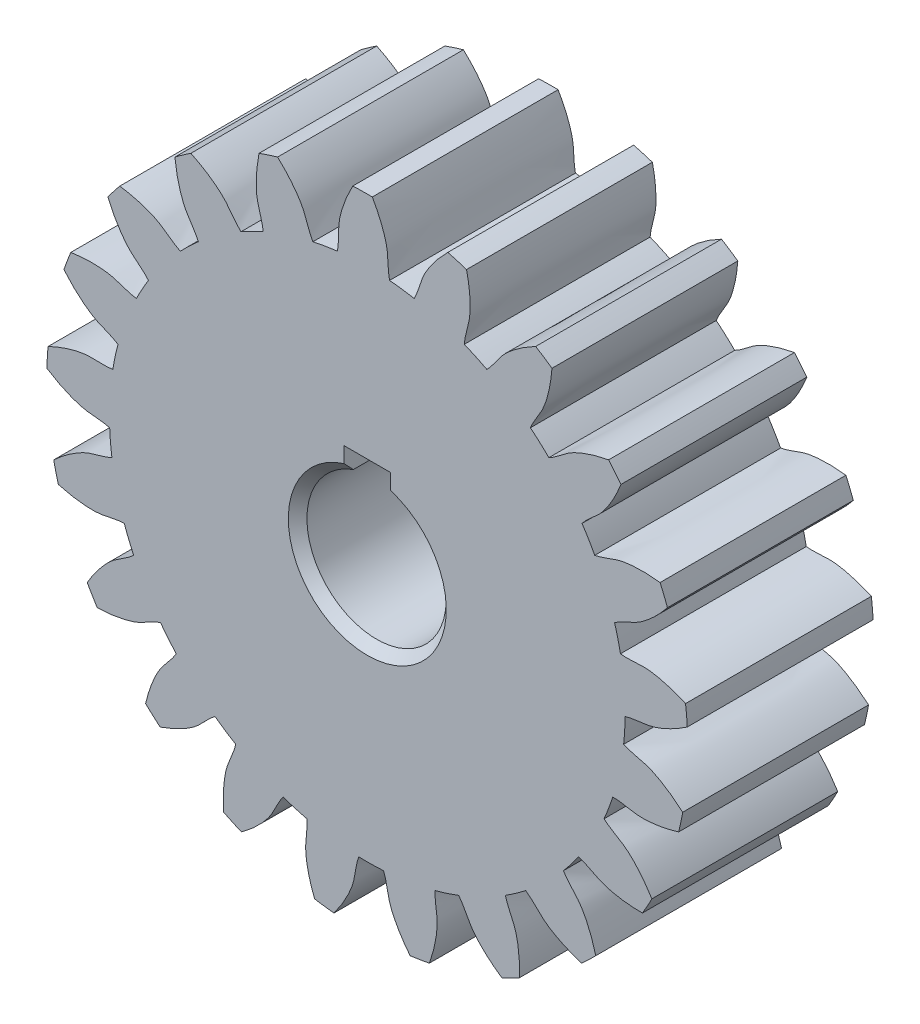
from build123d import *

# Parameters (mm, degrees)
SKETCH1_R           = 27.75
SKETCH1_R_2         = 7.5
BOSS_EXTRUDE1_DEPTH = 20
BOSS_EXTRUDE2_DEPTH = 20
CIRPATTERN1_COUNT   = 21
CHAMFER1_SIZE       = 1
CUT_EXTRUDE1_REACH  = 54.721
SKETCH3_W           = 5
SKETCH3_H           = 4.6


with BuildPart() as part:
    # Sketch1 → Boss-Extrude1 (new body)
    with BuildSketch(Plane.XY):
        Circle(SKETCH1_R)
        Circle(SKETCH1_R_2, mode=Mode.SUBTRACT)
    extrude(amount=BOSS_EXTRUDE1_DEPTH)

    # Sketch2 → Boss-Extrude2 (add)
    with BuildSketch(Plane.XY):
        with BuildLine():
            ThreePointArc((34.251201859, 4.135839847), (34.361284978, 3.090646322), (34.439480945, 2.042584688))
            add(Edge.make_bspline(
                [(34.439480945, 2.042584688), (33.828234224, 1.627292976), (32.886838359, 1.062288092), (31.572131173, 0.484167115), (30.003650173, -0.065068302), (28.663938322, -0.037592862), (27.748112829, -0.323627016)],
                knots=[0, 0, 0, 0, 0.308945746, 0.456629673, 0.599770858, 1, 1, 1, 1], degree=3))
            ThreePointArc((27.748112829, -0.323627016), (27.638424873, 2.48595465), (27.2449894, 5.270014477))
            add(Edge.make_bspline(
                [(34.251201859, 4.135839847), (33.57565822, 4.435390432), (32.548548574, 4.82333691), (31.151778933, 5.157572483), (29.510463248, 5.418100818), (28.197157458, 5.15199812), (27.2449894, 5.270014477)],
                knots=[0, 0, 0, 0, 0.308945746, 0.456629673, 0.599770858, 1, 1, 1, 1], degree=3))
        make_face()
    boss_extrude2 = extrude(amount=BOSS_EXTRUDE2_DEPTH)

    # CirPattern1: Boss-Extrude2 ×21 about axis
    cirpattern1_axis = Axis((0, 0, 20), (0, 0, -1))
    for i in range(1, CIRPATTERN1_COUNT):
        add(boss_extrude2.rotate(cirpattern1_axis, i * 360 / CIRPATTERN1_COUNT))

    # Chamfer1
    chamfer1_edges = [part.edges().sort_by_distance(p)[0] for p in [
        (-7.5, 0, 0),
        (-7.5, 0, 20),
    ]]
    chamfer(chamfer1_edges, length=CHAMFER1_SIZE)

    # Sketch3 → Cut-Extrude1 (cut, up to next)
    with BuildSketch(Plane.XY.offset(20), mode=Mode.PRIVATE) as cut_extrude1_sk1:
        with Locations((0, 7.5)):
            Rectangle(SKETCH3_W, SKETCH3_H)
    cut_extrude1_tool1 = extrude(cut_extrude1_sk1.sketch, amount=-CUT_EXTRUDE1_REACH, mode=Mode.PRIVATE) & part.part
    add(cut_extrude1_tool1.solids().sort_by_distance((0, 7.5, 20))[0], mode=Mode.SUBTRACT)


solid = part.part
